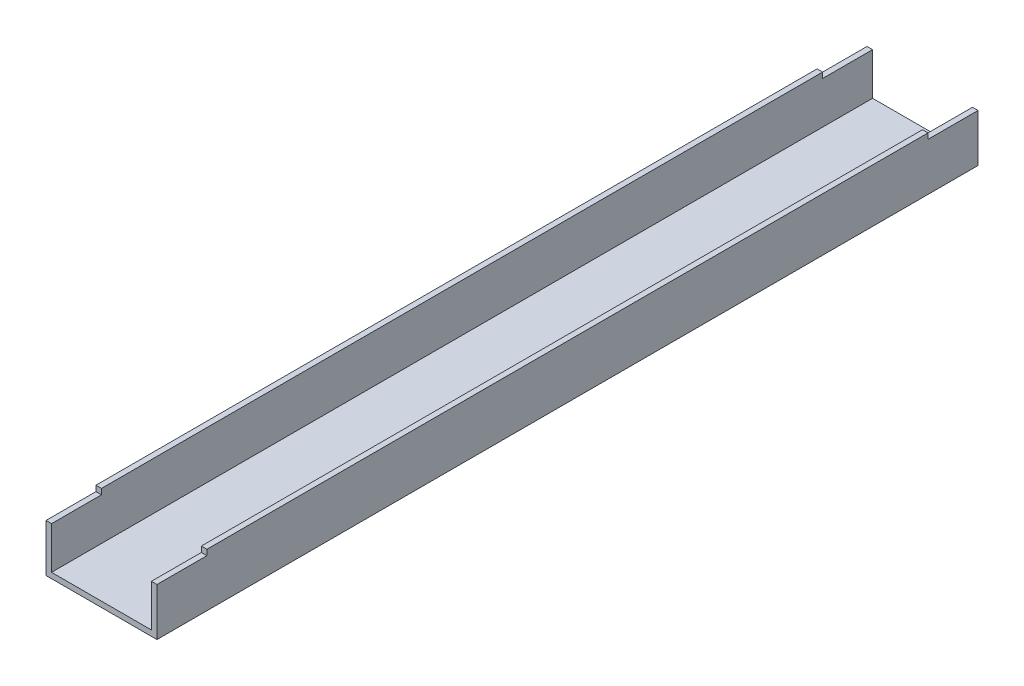
SolidWorks part; units mm, degrees
ref_plane "前视基准面" through (0, 0, 0) normal (0, 0, 1) x (1, 0, 0)
ref_plane "上视基准面" through (0, 0, 0) normal (0, 1, 0) x (1, 0, 0)
ref_plane "右视基准面" through (0, 0, 0) normal (1, 0, 0) x (0, 0, -1)
sketch "草图1" plane through (0, 0, 0) normal (0, 0, 1) x (1, 0, 0)
  line L0 (0, 0) -> (100, 0)
  line L1 (100, 0) -> (100, 48)
  line L2 (0, 0) -> (0, 48)
  line L3 (5, 5) -> (5, 48)
  line L4 (5, 5) -> (95, 5)
  line L5 (95, 5) -> (95, 48)
  line L6 (0, 48) -> (5, 48)
  line L7 (95, 48) -> (100, 48)
  dimension "D1" = 5
extrude "凸台-拉伸1" add sketch "草图1" along normal blind 740
sketch "草图2" plane through (0, 0, 0) normal (0, 0, -1) x (-1, 0, 0)
  line L0 (-100, 48) -> (-100, 43)
  line L1 (-100, 0) -> (-100, 48) construction
  line L2 (-100, 43) -> (0, 43)
  line L3 (0, 48) -> (0, 0) construction
  line L4 (0, 43) -> (0, 48)
  line L5 (0, 48) -> (-100, 48)
extrude "切除-拉伸1" cut sketch "草图2" against normal blind 45
sketch "草图3" plane through (0, 0, 740) normal (0, 0, 1) x (1, 0, 0)
  line L0 (0, 48) -> (0, 43)
  line L1 (0, 48) -> (0, 0) construction
  line L2 (0, 43) -> (100, 43)
  line L3 (100, 0) -> (100, 48) construction
  line L4 (100, 43) -> (100, 48)
  line L5 (100, 48) -> (0, 48)
extrude "切除-拉伸2" cut sketch "草图3" against normal blind 45
sketch "草图4" plane through (0, 0, 0) normal (0, -1, 0) x (1, 0, 0)
  line L0 (0, 370) -> (100, 370)
  line L1 (0, 740) -> (0, 0) construction
  line L2 (100, 740) -> (100, 0) construction
sketch "草图5" plane through (0, 0, 0) normal (-1, 0, 0) x (0, 0, 1)
  line L0 (370, 0) -> (370, 48)
  line L1 (740, 0) -> (0, 0) construction
  line L2 (695, 48) -> (45, 48) construction
sketch "草图6" plane through (0, 0, 0) normal (0, 0, -1) x (-1, 0, 0)
  line L16 (-95, 43) -> (-100, 43)
  line L17 (-100, 43) -> (-100, 0)
  line L18 (-100, 0) -> (0, 0)
  line L19 (0, 0) -> (0, 43)
  line L20 (0, 43) -> (-5, 43)
  line L21 (-5, 43) -> (-5, 5)
  line L22 (-5, 5) -> (-95, 5)
  line L23 (-95, 5) -> (-95, 43)
  line L24 (-95, 43) -> (-100, 43)
  line L25 (-100, 43) -> (-100, 0)
  line L26 (-100, 0) -> (0, 0)
  line L27 (0, 0) -> (0, 43)
  line L28 (0, 43) -> (-5, 43)
  line L29 (-5, 43) -> (-5, 5)
  line L30 (-5, 5) -> (-95, 5)
  line L31 (-95, 5) -> (-95, 43)
  dimension "D1" = 0
extrude "切除-拉伸3" cut sketch "草图6" against normal blind 25
sketch "草图7" plane through (0, 0, 740) normal (0, 0, 1) x (1, 0, 0)
  line L16 (100, 0) -> (100, 43)
  line L17 (100, 43) -> (95, 43)
  line L18 (95, 43) -> (95, 5)
  line L19 (95, 5) -> (5, 5)
  line L20 (5, 5) -> (5, 43)
  line L21 (5, 43) -> (0, 43)
  line L22 (0, 43) -> (0, 0)
  line L23 (0, 0) -> (100, 0)
  line L24 (100, 0) -> (100, 43)
  line L25 (100, 43) -> (95, 43)
  line L26 (95, 43) -> (95, 5)
  line L27 (95, 5) -> (5, 5)
  line L28 (5, 5) -> (5, 43)
  line L29 (5, 43) -> (0, 43)
  line L30 (0, 43) -> (0, 0)
  line L31 (0, 0) -> (100, 0)
  dimension "D1" = 0
extrude "切除-拉伸4" cut sketch "草图7" against normal blind 25
sketch "草图8" plane through (0, 0, 695) normal (0, 0, 1) x (1, 0, 0)
  line L8 (95, 48) -> (95, 43)
  line L9 (95, 43) -> (100, 43)
  line L10 (100, 43) -> (100, 48)
  line L11 (100, 48) -> (95, 48)
  line L12 (95, 48) -> (95, 43)
  line L13 (95, 43) -> (100, 43)
  line L14 (100, 43) -> (100, 48)
  line L15 (100, 48) -> (95, 48)
  line L20 (5, 43) -> (5, 48)
  line L21 (5, 48) -> (0, 48)
  line L22 (0, 48) -> (0, 43)
  line L23 (0, 43) -> (5, 43)
  line L24 (5, 43) -> (5, 48)
  line L25 (5, 48) -> (0, 48)
  line L26 (0, 48) -> (0, 43)
  line L27 (0, 43) -> (5, 43)
  dimension "D1" = 0
  dimension "D2" = 0
extrude "切除-拉伸5" cut sketch "草图8" against normal blind 25
sketch "草图9" plane through (0, 0, 45) normal (0, 0, -1) x (-1, 0, 0)
  line L8 (-5, 48) -> (-5, 43)
  line L9 (-5, 43) -> (0, 43)
  line L10 (0, 43) -> (0, 48)
  line L11 (0, 48) -> (-5, 48)
  line L12 (-5, 48) -> (-5, 43)
  line L13 (-5, 43) -> (0, 43)
  line L14 (0, 43) -> (0, 48)
  line L15 (0, 48) -> (-5, 48)
  line L20 (-95, 43) -> (-95, 48)
  line L21 (-95, 48) -> (-100, 48)
  line L22 (-100, 48) -> (-100, 43)
  line L23 (-100, 43) -> (-95, 43)
  line L24 (-95, 43) -> (-95, 48)
  line L25 (-95, 48) -> (-100, 48)
  line L26 (-100, 48) -> (-100, 43)
  line L27 (-100, 43) -> (-95, 43)
  dimension "D1" = 0
  dimension "D2" = 0
extrude "切除-拉伸6" cut sketch "草图9" against normal blind 25
sketch "草图10" plane through (0, 0, 25) normal (0, 0, -1) x (-1, 0, 0)
  line L16 (-95, 5) -> (-95, 43)
  line L17 (-95, 43) -> (-100, 43)
  line L18 (-100, 43) -> (-100, 0)
  line L19 (-100, 0) -> (0, 0)
  line L20 (0, 0) -> (0, 43)
  line L21 (0, 43) -> (-5, 43)
  line L22 (-5, 43) -> (-5, 5)
  line L23 (-5, 5) -> (-95, 5)
  line L24 (-95, 5) -> (-95, 43)
  line L25 (-95, 43) -> (-100, 43)
  line L26 (-100, 43) -> (-100, 0)
  line L27 (-100, 0) -> (0, 0)
  line L28 (0, 0) -> (0, 43)
  line L29 (0, 43) -> (-5, 43)
  line L30 (-5, 43) -> (-5, 5)
  line L31 (-5, 5) -> (-95, 5)
  dimension "D1" = 0
extrude "凸台-拉伸2" add sketch "草图10" along normal blind 25
sketch "草图11" plane through (0, 0, 70) normal (0, 0, -1) x (-1, 0, 0)
  line L8 (0, 48) -> (-5, 48)
  line L9 (-5, 48) -> (-5, 43)
  line L10 (-5, 43) -> (0, 43)
  line L11 (0, 43) -> (0, 48)
  line L12 (0, 48) -> (-5, 48)
  line L13 (-5, 48) -> (-5, 43)
  line L14 (-5, 43) -> (0, 43)
  line L15 (0, 43) -> (0, 48)
  line L20 (-100, 43) -> (-95, 43)
  line L21 (-95, 43) -> (-95, 48)
  line L22 (-95, 48) -> (-100, 48)
  line L23 (-100, 48) -> (-100, 43)
  line L24 (-100, 43) -> (-95, 43)
  line L25 (-95, 43) -> (-95, 48)
  line L26 (-95, 48) -> (-100, 48)
  line L27 (-100, 48) -> (-100, 43)
  dimension "D1" = 0
  dimension "D2" = 0
extrude "凸台-拉伸3" add sketch "草图11" along normal blind 25
sketch "草图12" plane through (0, 0, 715) normal (0, 0, 1) x (1, 0, 0)
  line L16 (0, 0) -> (100, 0)
  line L17 (100, 0) -> (100, 43)
  line L18 (100, 43) -> (95, 43)
  line L19 (95, 43) -> (95, 5)
  line L20 (95, 5) -> (5, 5)
  line L21 (5, 5) -> (5, 43)
  line L22 (5, 43) -> (0, 43)
  line L23 (0, 43) -> (0, 0)
  line L24 (0, 0) -> (100, 0)
  line L25 (100, 0) -> (100, 43)
  line L26 (100, 43) -> (95, 43)
  line L27 (95, 43) -> (95, 5)
  line L28 (95, 5) -> (5, 5)
  line L29 (5, 5) -> (5, 43)
  line L30 (5, 43) -> (0, 43)
  line L31 (0, 43) -> (0, 0)
  dimension "D1" = 0
extrude "凸台-拉伸4" add sketch "草图12" along normal blind 25
sketch "草图13" plane through (0, 0, 670) normal (0, 0, 1) x (1, 0, 0)
  line L8 (0, 43) -> (5, 43)
  line L9 (5, 43) -> (5, 48)
  line L10 (5, 48) -> (0, 48)
  line L11 (0, 48) -> (0, 43)
  line L12 (0, 43) -> (5, 43)
  line L13 (5, 43) -> (5, 48)
  line L14 (5, 48) -> (0, 48)
  line L15 (0, 48) -> (0, 43)
  line L20 (100, 48) -> (95, 48)
  line L21 (95, 48) -> (95, 43)
  line L22 (95, 43) -> (100, 43)
  line L23 (100, 43) -> (100, 48)
  line L24 (100, 48) -> (95, 48)
  line L25 (95, 48) -> (95, 43)
  line L26 (95, 43) -> (100, 43)
  line L27 (100, 43) -> (100, 48)
  dimension "D1" = 0
  dimension "D2" = 0
extrude "凸台-拉伸5" add sketch "草图13" along normal blind 25
